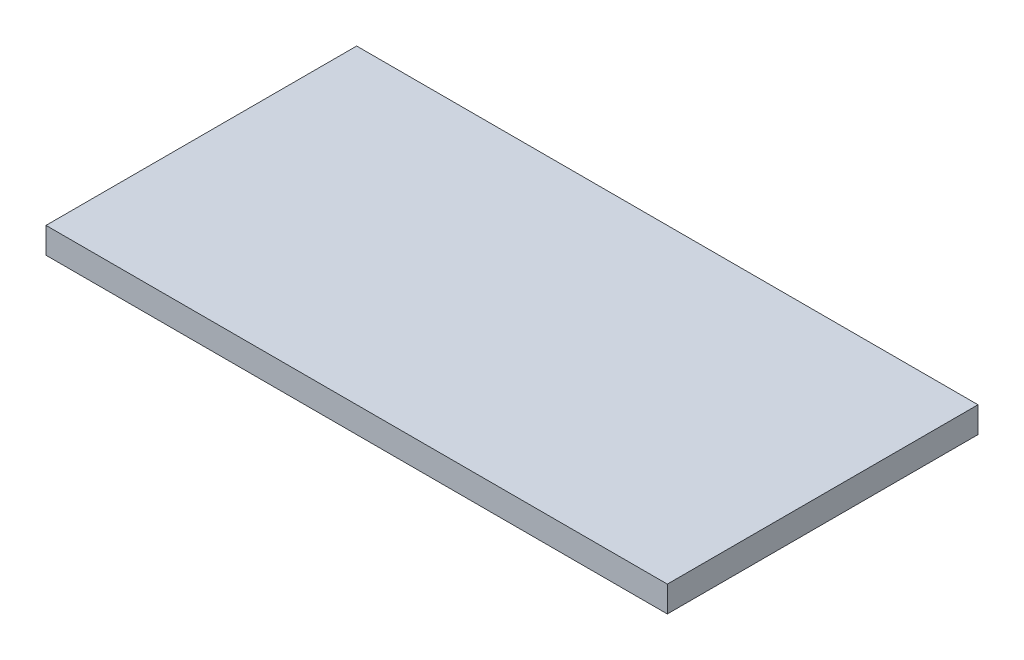
SolidWorks part; units mm, degrees
ref_plane "Front Plane" through (0, 0, 0) normal (0, 0, 1) x (1, 0, 0)
ref_plane "Top Plane" through (0, 0, 0) normal (0, 1, 0) x (1, 0, 0)
ref_plane "Right Plane" through (0, 0, 0) normal (1, 0, 0) x (0, 0, -1)
sketch "Sketch1" plane through (0, 0, 0) normal (0, 1, 0) x (1, 0, 0)
  line L1 (-60, 30) -> (60, 30)
  line L2 (-60, 30) -> (-60, -30)
  line L3 (-60, -30) -> (60, -30)
  line L4 (60, 30) -> (60, -30)
  line L5 (-60, 30) -> (60, -30) construction
  line L6 (-60, -30) -> (60, 30) construction
  point P0 (0, 0)
  dimension "D1" = 120
  dimension "D2" = 60
extrude "Boss-Extrude1" add sketch "Sketch1" along normal blind 5
